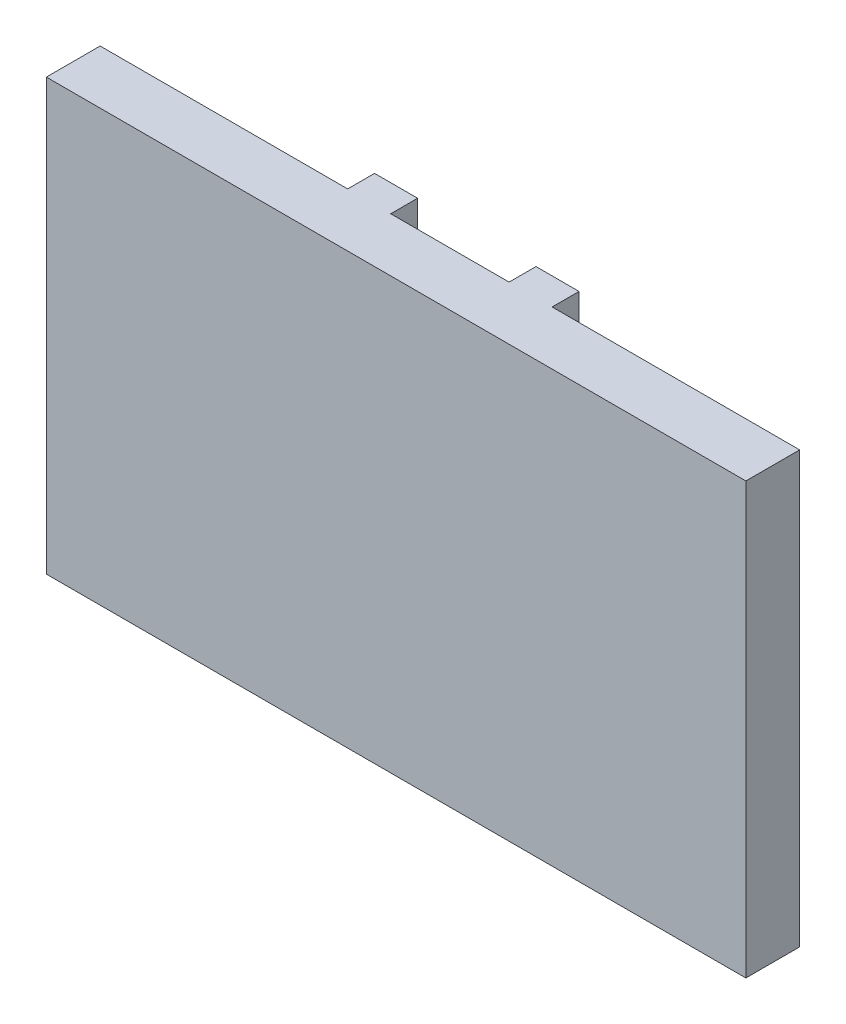
SolidWorks part; units mm, degrees
ref_plane "Front Plane" through (0, 0, 0) normal (0, 0, 1) x (1, 0, 0)
ref_plane "Top Plane" through (0, 0, 0) normal (0, 1, 0) x (1, 0, 0)
ref_plane "Right Plane" through (0, 0, 0) normal (1, 0, 0) x (0, 0, -1)
sketch "Sketch3" plane through (0, 0, 0) normal (0, 0, 1) x (1, 0, 0)
  line L0 (720, 319) -> (720, 119) construction
  line L1 (690, 319) -> (750, 319) construction
  line L3 (785, 159) -> (655, 159)
  line L8 (785, 159) -> (785, 79)
  line L9 (785, 79) -> (655, 79)
  line L10 (655, 159) -> (655, 79)
  line L11 (785, 159) -> (655, 79) construction
  line L12 (785, 79) -> (655, 159) construction
  dimension "D1" = 80
  dimension "D2" = 130
  dimension "D3" = 200
extrude "Boss-Extrude1" add sketch "Sketch3" along normal blind 10
sketch "Sketch4" plane through (0, 0, 0) normal (0, 0, -1) x (-1, 0, 0)
  line L0 (-739, 159) -> (-731, 159)
  line L1 (-785, 159) -> (-655, 159) construction
  line L2 (-739, 79) -> (-731, 79)
  line L3 (-655, 79) -> (-785, 79) construction
  line L4 (-739, 299) -> (-739, -299)
  line L5 (-731, 299) -> (-739, 299)
  line L6 (-731, -299) -> (-731, 299)
  line L7 (-739, -299) -> (-731, -299)
  line L8 (-739, 159) -> (-739, 79)
  line L10 (-731, 79) -> (-731, 159)
  line L12 (-709, 79) -> (-701, 79)
  line L13 (-709, 159) -> (-701, 159)
  line L16 (-709, 299) -> (-709, -299)
  line L17 (-701, 299) -> (-709, 299)
  line L18 (-701, -299) -> (-701, 299)
  line L19 (-709, -299) -> (-701, -299)
  line L20 (-709, 159) -> (-709, 79)
  line L22 (-701, 79) -> (-701, 159)
  dimension "D2" = 0
  dimension "D1" = 0
extrude "Boss-Extrude2" add sketch "Sketch4" along normal up to surface (5 mm away)
